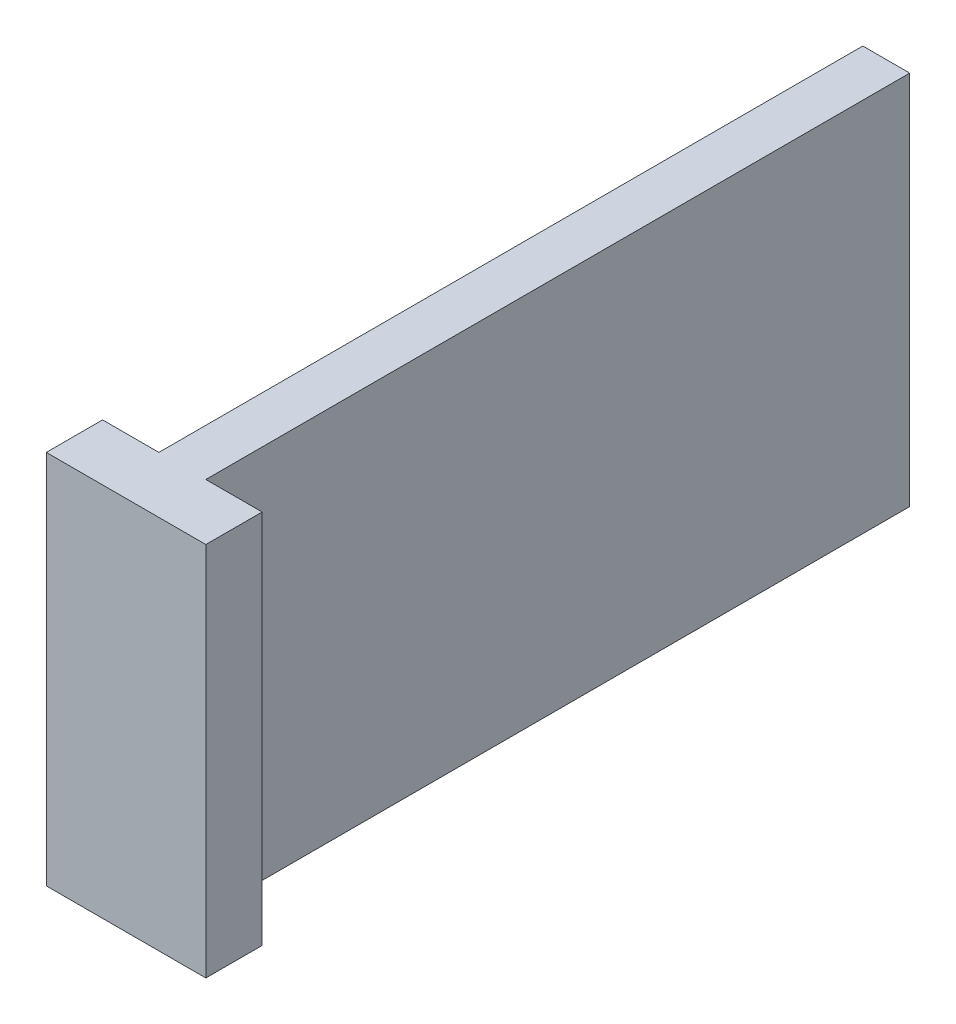
from build123d import *

# Parameters (mm, degrees)
SKETCH_1_W      = 150
SKETCH_1_H      = 80
EXTRUDE_1_DEPTH = 5
SKETCH_2_W      = 22
SKETCH_2_H      = 80
EXTRUDE_2_DEPTH = 12


with BuildPart() as part:
    # 草图1 → 凸台-拉伸1 (new, symmetric)
    with BuildSketch(Plane(origin=(0, 0, 0), x_dir=(0, 0, -1), z_dir=(1, 0, 0))):
        Rectangle(SKETCH_1_W, SKETCH_1_H)
    extrude(amount=EXTRUDE_1_DEPTH, both=True)

    # 草图2 → 凸台-拉伸2 (add)
    with BuildSketch(Plane.XY.offset(75)):
        with Locations((6, 0)):
            Rectangle(SKETCH_2_W, SKETCH_2_H)
    extrude_2 = extrude(amount=EXTRUDE_2_DEPTH)

    # 镜向1: 凸台-拉伸2 across plane
    add(extrude_2.mirror(Plane(origin=(0, 0, 0), x_dir=(0, 0, 1), z_dir=(1, 0, 0))))


solid = part.part
